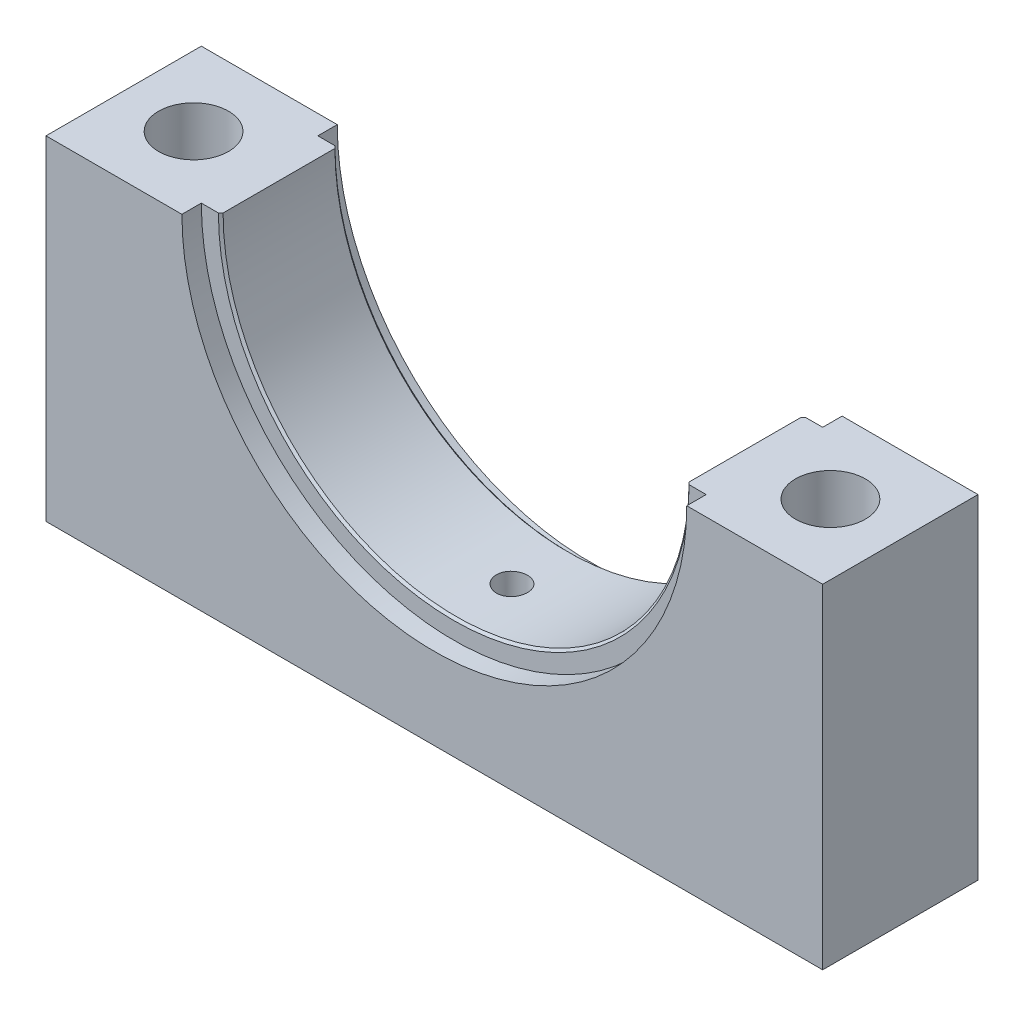
from build123d import *

# Parameters (mm, degrees)
BOSS_EXTRUDE1_DEPTH = 20
SKETCH2_R           = 32.5
CUT_EXTRUDE1_DEPTH  = 2.5
CUT_EXTRUDE2_START  = -2.5
SKETCH3_R           = 32.5
CUT_EXTRUDE2_DEPTH  = 2.5
CHAMFER1_SIZE       = 0.3
HOLE1_D             = 9
HOLE2_D             = 4
HOLE2_DEPTH         = 34


with BuildPart() as part:
    # Sketch1 → Boss-Extrude1 (new body)
    with BuildSketch(Plane.XY):
        with BuildLine():
            Line((-50, 0), (-30, 0))
            ThreePointArc((-30, 0), (0, -30), (30, 0))
            Line((30, 0), (50, 0))
            Line((50, 0), (50, -43))
            Line((50, -43), (-50, -43))
            Line((-50, -43), (-50, 0))
        make_face()
    extrude(amount=BOSS_EXTRUDE1_DEPTH)

    # Sketch2 → Cut-Extrude1 (cut)
    with BuildSketch(Plane.XY.offset(20)):
        Circle(SKETCH2_R)
    extrude(amount=-CUT_EXTRUDE1_DEPTH, mode=Mode.SUBTRACT)

    # Sketch3 → Cut-Extrude2 (cut)
    with BuildSketch(Plane(origin=(0, 0, 0), x_dir=(-1, 0, 0), z_dir=(0, 0, -1)).offset(CUT_EXTRUDE2_START)):
        Circle(SKETCH3_R)
    extrude(amount=CUT_EXTRUDE2_DEPTH, mode=Mode.SUBTRACT)

    # Chamfer1
    chamfer1_edges = [part.edges().sort_by_distance(p)[0] for p in [
        (0, -30, 17.5),
        (0, -30, 2.5),
    ]]
    chamfer(chamfer1_edges, length=CHAMFER1_SIZE)

    # Hole1 (through all)
    with Locations(Plane(origin=(0, 0, 0), x_dir=(1, 0, 0), z_dir=(0, 1, 0))):
        with Locations((-41, -10), (41, -10)):
            Hole(HOLE1_D / 2)

    # Hole2
    with Locations(Plane(origin=(0, 0, 0), x_dir=(1, 0, 0), z_dir=(0, 1, 0))):
        with Locations((0, -10)):
            Hole(HOLE2_D / 2, depth=HOLE2_DEPTH)


solid = part.part
